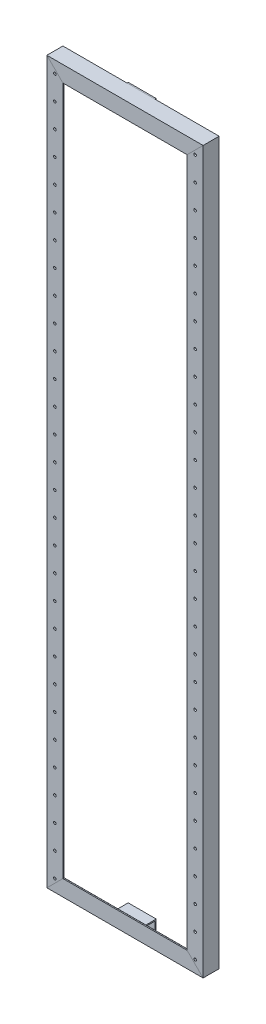
SolidWorks part; units mm, degrees
material "1023 碳钢板 (SS)"
ref_plane "前视基准面" through (0, 0, 0) normal (0, 0, 1) x (1, 0, 0)
ref_plane "上视基准面" through (0, 0, 0) normal (0, 1, 0) x (1, 0, 0)
ref_plane "右视基准面" through (0, 0, 0) normal (1, 0, 0) x (0, 0, -1)
sketch "草图1" plane through (0, 0, 0) normal (0, 0, 1) x (1, 0, 0)
  line L1 (195, -900) -> (-195, -900)
  line L2 (195, -900) -> (195, 900)
  line L3 (195, 900) -> (-195, 900)
  line L4 (-195, -900) -> (-195, 900)
  line L5 (195, -900) -> (-195, 900) construction
  line L6 (195, 900) -> (-195, -900) construction
  point P0 (0, 0)
  dimension "D1" = 1800
  dimension "D2" = 390
other "结构构件1"
ref_plane "基准面1" through (195, -900, 0) normal (0, 1, 0) x (-1, 0, 0)
sketch "Sketch1" plane through (195, -900, 0) normal (0, 1, 0) x (-1, 0, 0)
  line L0 (40, 0) -> (0, 0)
  line L1 (0, 0) -> (0, -40)
  line L2 (38.6667, -4) -> (9, -4)
  line L3 (4, -9) -> (4, -38.6667)
  line L4 (40, 0) -> (40, -2.6667)
  line L5 (0, -40) -> (2.6667, -40)
  arc A0 (40, -2.6667) -> (38.6667, -4) centre (38.6667, -2.6667) cw
  arc A1 (2.6667, -40) -> (4, -38.6667) centre (2.6667, -38.6667) ccw
  arc A2 (9, -4) -> (4, -9) centre (9, -9) ccw
  point P2 (20, 0)
  point P13 (0, -20)
  point P15 (0, 0)
  dimension "r1" = 1.3333
  dimension "r" = 5
  dimension "b" = 40
  dimension "d" = 4
sketch "草图2" plane through (0, 0, 0) normal (0, 0, 1) x (1, 0, 0)
  line L0 (195, 900) -> (195, -900) construction
  line L1 (-195, 900) -> (195, 900) construction
  line L2 (0, 900) -> (0, 731.247) construction
  circle A0 centre (175, 870) radius 3.25
  circle A1 centre (-175, 870) radius 3.25
  circle A2 centre (-175, 810) radius 3.25
  circle A3 centre (175, 810) radius 3.25
  circle A4 centre (-175, 750) radius 3.25
  circle A5 centre (175, 750) radius 3.25
  circle A6 centre (-175, 690) radius 3.25
  circle A7 centre (175, 690) radius 3.25
  circle A8 centre (-175, 630) radius 3.25
  circle A9 centre (175, 630) radius 3.25
  circle A10 centre (-175, 570) radius 3.25
  circle A11 centre (175, 570) radius 3.25
  circle A12 centre (-175, 510) radius 3.25
  circle A13 centre (175, 510) radius 3.25
  circle A14 centre (-175, 450) radius 3.25
  circle A15 centre (175, 450) radius 3.25
  circle A16 centre (-175, 390) radius 3.25
  circle A17 centre (175, 390) radius 3.25
  circle A18 centre (-175, 330) radius 3.25
  circle A19 centre (175, 330) radius 3.25
  circle A20 centre (-175, 270) radius 3.25
  circle A21 centre (175, 270) radius 3.25
  circle A22 centre (-175, 210) radius 3.25
  circle A23 centre (175, 210) radius 3.25
  circle A24 centre (-175, 150) radius 3.25
  circle A25 centre (175, 150) radius 3.25
  circle A26 centre (-175, 90) radius 3.25
  circle A27 centre (175, 90) radius 3.25
  circle A28 centre (-175, 30) radius 3.25
  circle A29 centre (175, 30) radius 3.25
  circle A30 centre (-175, -30) radius 3.25
  circle A31 centre (175, -30) radius 3.25
  circle A32 centre (-175, -90) radius 3.25
  circle A33 centre (175, -90) radius 3.25
  circle A34 centre (-175, -150) radius 3.25
  circle A35 centre (175, -150) radius 3.25
  circle A36 centre (-175, -210) radius 3.25
  circle A37 centre (175, -210) radius 3.25
  circle A38 centre (-175, -270) radius 3.25
  circle A39 centre (175, -270) radius 3.25
  circle A40 centre (-175, -330) radius 3.25
  circle A41 centre (175, -330) radius 3.25
  circle A42 centre (-175, -390) radius 3.25
  circle A43 centre (175, -390) radius 3.25
  circle A44 centre (-175, -450) radius 3.25
  circle A45 centre (175, -450) radius 3.25
  circle A46 centre (-175, -510) radius 3.25
  circle A47 centre (175, -510) radius 3.25
  circle A48 centre (-175, -570) radius 3.25
  circle A49 centre (175, -570) radius 3.25
  circle A50 centre (-175, -630) radius 3.25
  circle A51 centre (175, -630) radius 3.25
  circle A52 centre (-175, -690) radius 3.25
  circle A53 centre (175, -690) radius 3.25
  circle A54 centre (-175, -750) radius 3.25
  circle A55 centre (175, -750) radius 3.25
  circle A56 centre (-175, -810) radius 3.25
  circle A57 centre (175, -810) radius 3.25
  circle A58 centre (-175, -870) radius 3.25
  circle A59 centre (175, -870) radius 3.25
  dimension "D1" = 6.5
  dimension "D2" = 20
  dimension "D3" = 30
  dimension "D4" = 30
extrude "切除-拉伸1" cut sketch "草图2" against normal up to next (4 mm away)
sketch "草图3" plane through (0, 0, 0) normal (1, 0, 0) x (0, 0, -1)
  line L0 (0, 0) -> (347.1691, 0) construction
  line L1 (3, -874) -> (3, -877)
  line L2 (40, -900) -> (43, -900)
  line L3 (3, 874) -> (43, 874)
  line L4 (43, 900) -> (43, 874)
  line L5 (3, -874) -> (43, -874)
  line L7 (3, 877) -> (40, 877)
  line L8 (40, 900) -> (40, 877)
  line L9 (3, -877) -> (40, -877)
  line L10 (40, -900) -> (40, -877)
  line L11 (43, -900) -> (43, -874)
  line L13 (3, 877) -> (3, 874)
  line L14 (40, 900) -> (43, 900)
  line L15 (0, 900) -> (0, -900) construction
  dimension "D1" = 40
  dimension "D2" = 40
  dimension "D3" = 26
  dimension "D4" = 26
  dimension "D5" = 3
extrude "凸台-拉伸1" add sketch "草图3" along normal mid plane 70 separate body
